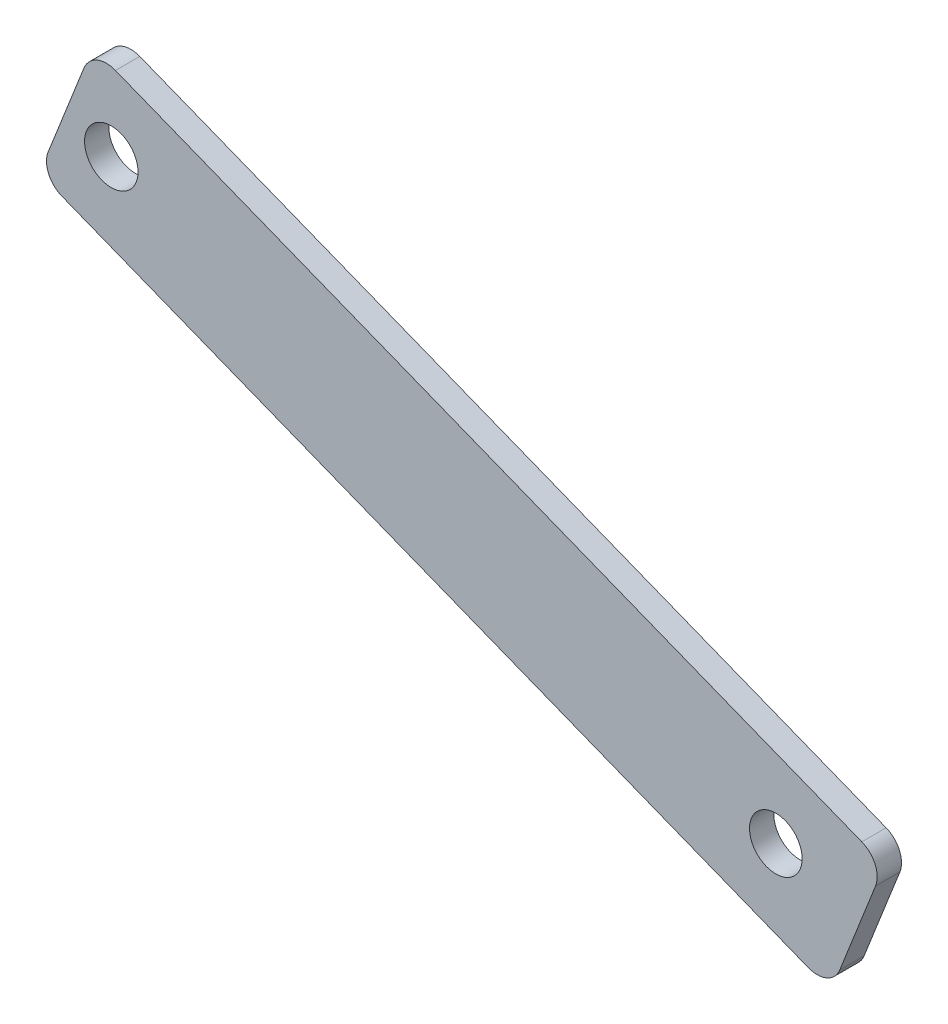
from build123d import *

# Parameters (mm, degrees)
EXTRUDE_START   = 40
SKETCH_1_R      = 11
SKETCH_1_R_2    = 10.824525282
EXTRUDE_1_DEPTH = 10


with BuildPart() as part:
    # 草图1 → 凸台-拉伸1 (new body)
    with BuildSketch(Plane.XY.offset(-1083.237354735).offset(EXTRUDE_START)):
        with BuildLine():
            Line((-135.515744069, 493.626345969), (171.40128741, 372.374806646))
            ThreePointArc((171.40128741, 372.374806646), (176.901571064, 367.052633829), (177.027514445, 359.40000147))
            Line((177.027514445, 359.40000147), (162.330358163, 322.197937048))
            ThreePointArc((162.330358163, 322.197937048), (157.008185347, 316.697653394), (149.355552988, 316.571710013))
            Line((149.355552988, 316.571710013), (-157.561478491, 437.823249336))
            ThreePointArc((-157.561478491, 437.823249336), (-163.061762145, 443.145422153), (-163.187705526, 450.798054512))
            Line((-163.187705526, 450.798054512), (-148.490549245, 488.000118934))
            ThreePointArc((-148.490549245, 488.000118934), (-143.168376428, 493.500402588), (-135.515744069, 493.626345969))
        make_face()
        with Locations((-137.238095175, 462.050508582)):
            Circle(SKETCH_1_R, mode=Mode.SUBTRACT)
        with Locations((136.038969551, 354.088872827)):
            Circle(SKETCH_1_R_2, mode=Mode.SUBTRACT)
    extrude(amount=EXTRUDE_1_DEPTH)


solid = part.part
